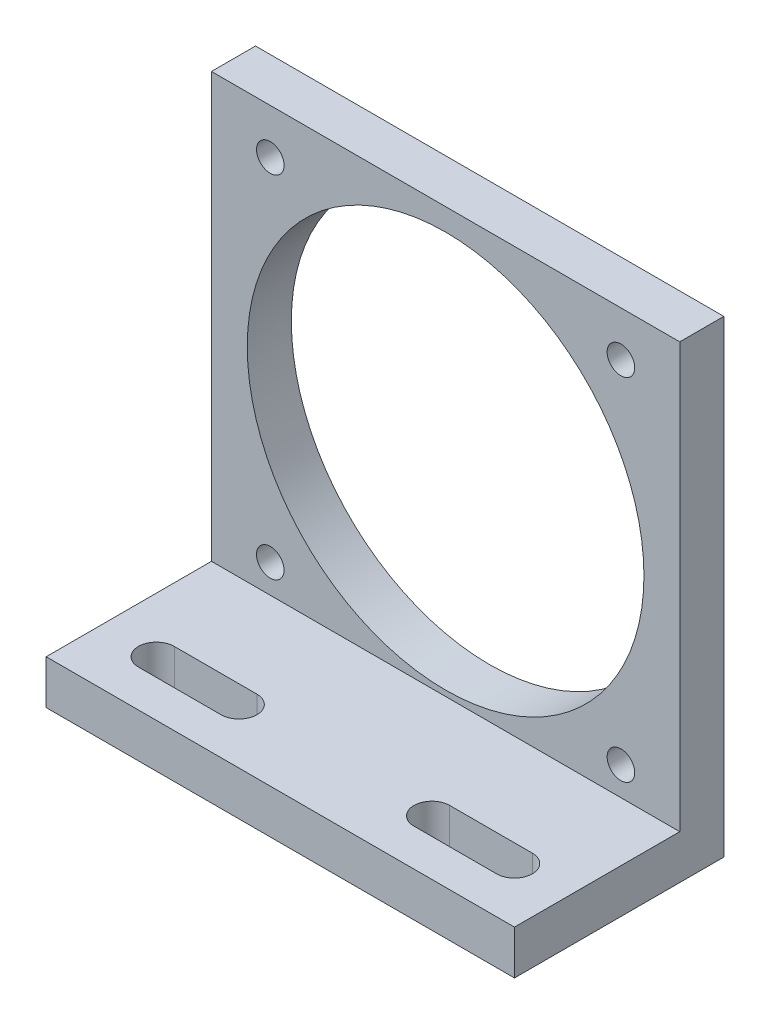
from build123d import *

# Parameters (mm, degrees)
SKETCH_1_W          = 85
SKETCH_1_H          = 85
SKETCH_1_R          = 36
EXTRUDE_1_DEPTH     = 4
HOLE_WIZARD_M6_1_D  = 5
SKETCH_4_W          = 85
SKETCH_4_H          = 8
EXTRUDE_2_DEPTH     = 30
CUT_EXTRUDE_1_DEPTH = 95.293425009


with BuildPart() as part:
    # 草图1 → 凸台-拉伸1 (new, symmetric)
    with BuildSketch(Plane.XY):
        Rectangle(SKETCH_1_W, SKETCH_1_H)
        with Locations((0, 2.5)):
            Circle(SKETCH_1_R, mode=Mode.SUBTRACT)
    extrude(amount=EXTRUDE_1_DEPTH, both=True)

    # M6 螺纹孔1 (through all)
    with Locations(Plane(origin=(-31.819805153, 34.319805153, 4), x_dir=(1, 0, 0), z_dir=(0, 0, 1))):
        with Locations((0, 0), (63.639610306, -63.639610306), (0, -63.639610306), (63.639610306, 0)):
            Hole(HOLE_WIZARD_M6_1_D / 2)

    # 草图4 → 凸台-拉伸2 (add)
    with BuildSketch(Plane.XY.offset(4)):
        with Locations((0, -38.5)):
            Rectangle(SKETCH_4_W, SKETCH_4_H)
    extrude(amount=EXTRUDE_2_DEPTH)

    # 草图5 → 切除-拉伸1 (cut, through all)
    with BuildSketch(Plane(origin=(0, -34.5, 0), x_dir=(1, 0, 0), z_dir=(0, 1, 0))):
        with BuildLine():
            Line((-32.5, -20.75), (-17.5, -20.75))
            ThreePointArc((-17.5, -20.75), (-14.25, -24), (-17.5, -27.25))
            Line((-17.5, -27.25), (-32.5, -27.25))
            ThreePointArc((-32.5, -27.25), (-35.75, -24), (-32.5, -20.75))
        make_face()
        with BuildLine():
            Line((17.5, -20.75), (32.5, -20.75))
            ThreePointArc((32.5, -20.75), (35.75, -24), (32.5, -27.25))
            Line((32.5, -27.25), (17.5, -27.25))
            ThreePointArc((17.5, -27.25), (14.25, -24), (17.5, -20.75))
        make_face()
    extrude(amount=-CUT_EXTRUDE_1_DEPTH, mode=Mode.SUBTRACT)


solid = part.part
